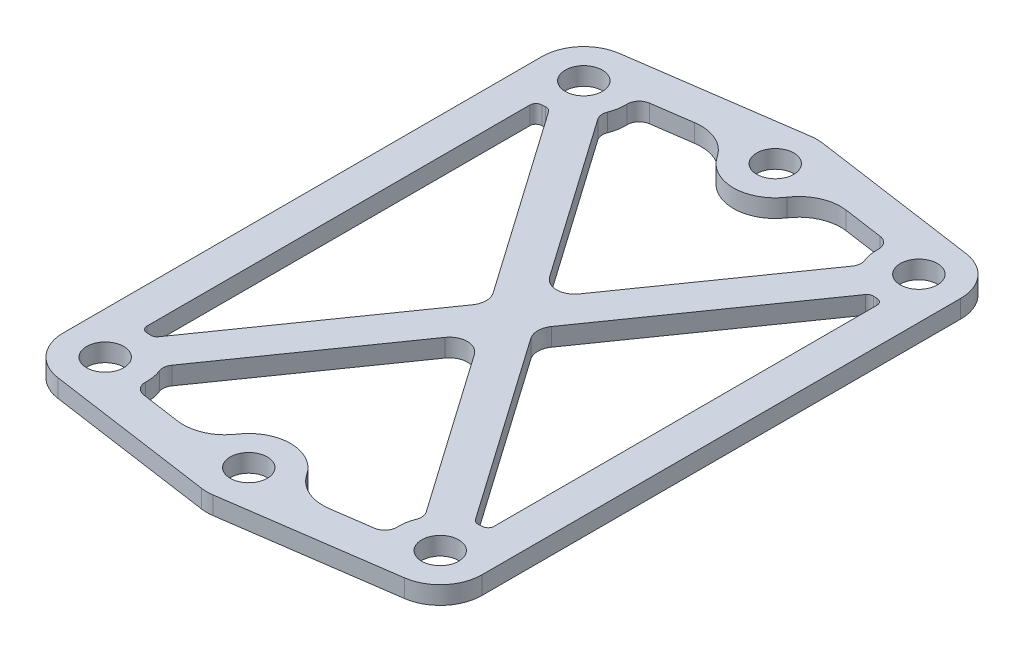
SolidWorks part; units mm, degrees
material "Thornel Mat VMA"
ref_plane "前视基准面" through (0, 0, 0) normal (0, 0, 1) x (1, 0, 0)
ref_plane "上视基准面" through (0, 0, 0) normal (0, 1, 0) x (1, 0, 0)
ref_plane "右视基准面" through (0, 0, 0) normal (1, 0, 0) x (0, 0, -1)
other "Configuration Table"
sketch "草图1" plane through (0, 0, 0) normal (0, 1, 0) x (1, 0, 0)
  line L0 (0, 0) -> (26.6949, 0) construction
  line L1 (-14, 20) -> (14, 20) construction
  line L2 (-14, 20) -> (-14, -20) construction
  line L3 (-14, -20) -> (14, -20) construction
  line L4 (14, 20) -> (14, -20) construction
  line L5 (-14, 20) -> (14, -20) construction
  line L6 (-14, -20) -> (14, 20) construction
  line L7 (0, 0) -> (0, 34.1992) construction
  line L8 (-14.5, 16.5359) -> (-14.5, -16.5359)
  line L11 (-17.5, 20) -> (-17.5, -20)
  line L14 (-14.495, 23.4648) -> (-0.495, 25.4648)
  line L15 (-10.6414, 20.9849) -> (-3.5, 22.0051)
  line L17 (-10.9577, 18.2696) -> (13.4154, -16.5492)
  line L20 (-13.4154, 16.5492) -> (10.9577, -18.2696)
  line L22 (-13.4154, -16.5492) -> (10.9577, 18.2696)
  line L23 (-10.9577, -18.2696) -> (13.4154, 16.5492)
  line L24 (-14.495, -23.4648) -> (-0.495, -25.4648)
  line L25 (-10.6414, -20.9849) -> (-3.5, -22.0051)
  line L26 (10.6414, -20.9849) -> (3.5, -22.0051)
  line L27 (14.495, -23.4648) -> (0.495, -25.4648)
  line L28 (14.495, 23.4648) -> (0.495, 25.4648)
  line L29 (17.5, 20) -> (17.5, -20)
  line L30 (10.6414, 20.9849) -> (3.5, 22.0051)
  line L31 (14.5, 16.5359) -> (14.5, -16.5359)
  circle A0 centre (14, 20) radius 1.55
  circle A1 centre (14, -20) radius 1.55
  circle A2 centre (-14, -20) radius 1.55
  circle A3 centre (-14, 20) radius 1.55
  circle A4 centre (0, 22) radius 1.55
  circle A5 centre (0, -22) radius 1.55
  circle A22 centre (-14, 20) radius 3.5
  circle A23 centre (0, 22) radius 3.5
  circle A24 centre (14, 20) radius 3.5
  circle A25 centre (14, -20) radius 3.5
  circle A26 centre (0, -22) radius 3.5
  circle A27 centre (-14, -20) radius 3.5
  point P0 (0, 0)
  dimension "D3" = 2
  dimension "D4" = 3.1
  dimension "D5" = 7
  dimension "D6" = 3
  dimension "D1" = 28
  dimension "D2" = 40
  dimension "D7" = 3
  dimension "D8" = 3
extrude "凸台-拉伸1" add sketch "草图1" along normal blind 1.5
fillet "圆角1" radius 0.5 8 edges at (-13.4154, 0.75, 16.5492) (-14.5, 0.75, 16.5359) (14.5, 0.75, 16.5359) (13.4154, 0.75, 16.5492) (14.5, 0.75, -16.5359) (13.4154, 0.75, -16.5492) (-13.4154, 0.75, -16.5492) (-14.5, 0.75, -16.5359)
fillet "圆角2" radius 1 8 edges at (10.9577, 0.75, 18.2696) (10.6414, 0.75, 20.9849) (-10.6414, 0.75, 20.9849) (-10.9577, 0.75, 18.2696) (10.9577, 0.75, -18.2696) (10.6414, 0.75, -20.9849) (-10.9577, 0.75, -18.2696) (-10.6414, 0.75, -20.9849)
fillet "圆角3" radius 1.5 4 edges at (0, 0.75, -2.6157) (1.831, 0.75, 0) (-1.831, 0.75, 0) (0, 0.75, 2.6157)
fillet "圆角4" radius 3.5 4 edges at (3.5, 0.75, -22.0051) (-3.5, 0.75, -22.0051) (3.5, 0.75, 22.0051) (-3.5, 0.75, 22.0051)
